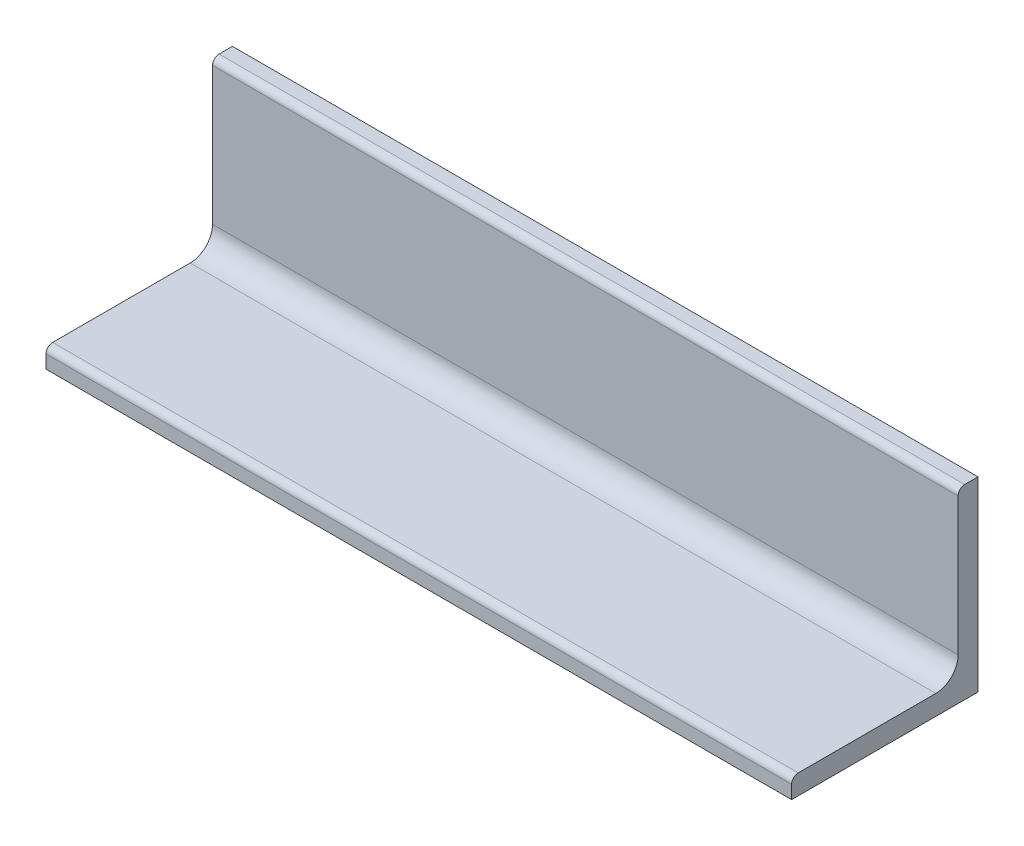
SolidWorks part; units mm, degrees
ref_plane "Front" through (0, 0, 0) normal (0, 0, 1) x (1, 0, 0)
ref_plane "Top" through (0, 0, 0) normal (0, 1, 0) x (1, 0, 0)
ref_plane "Right" through (0, 0, 0) normal (1, 0, 0) x (0, 0, -1)
other "Configuration Table"
sketch "Sketch1" plane through (0, 0, 0) normal (1, 0, 0) x (0, 1, 0)
  line L0 (0, 75) -> (0, 0)
  line L1 (0, 0) -> (75, 0)
  line L2 (8, 72.3333) -> (8, 17)
  line L3 (17, 8) -> (72.3333, 8)
  line L4 (0, 75) -> (5.3333, 75)
  line L5 (75, 0) -> (75, 5.3333)
  arc A0 (5.3333, 75) -> (8, 72.3333) centre (5.3333, 72.3333) cw
  arc A1 (75, 5.3333) -> (72.3333, 8) centre (72.3333, 5.3333) ccw
  arc A2 (8, 17) -> (17, 8) centre (17, 17) ccw
extrude "Base" add sketch "Sketch1" along normal blind 300
equation "\"r1@Sketch1\" = \"d@Sketch1\" / 3"
equation "\"d1@Sketch1\" = \"d@Sketch1\""
equation "\"b1@Sketch1\" = \"b@Sketch1\""
